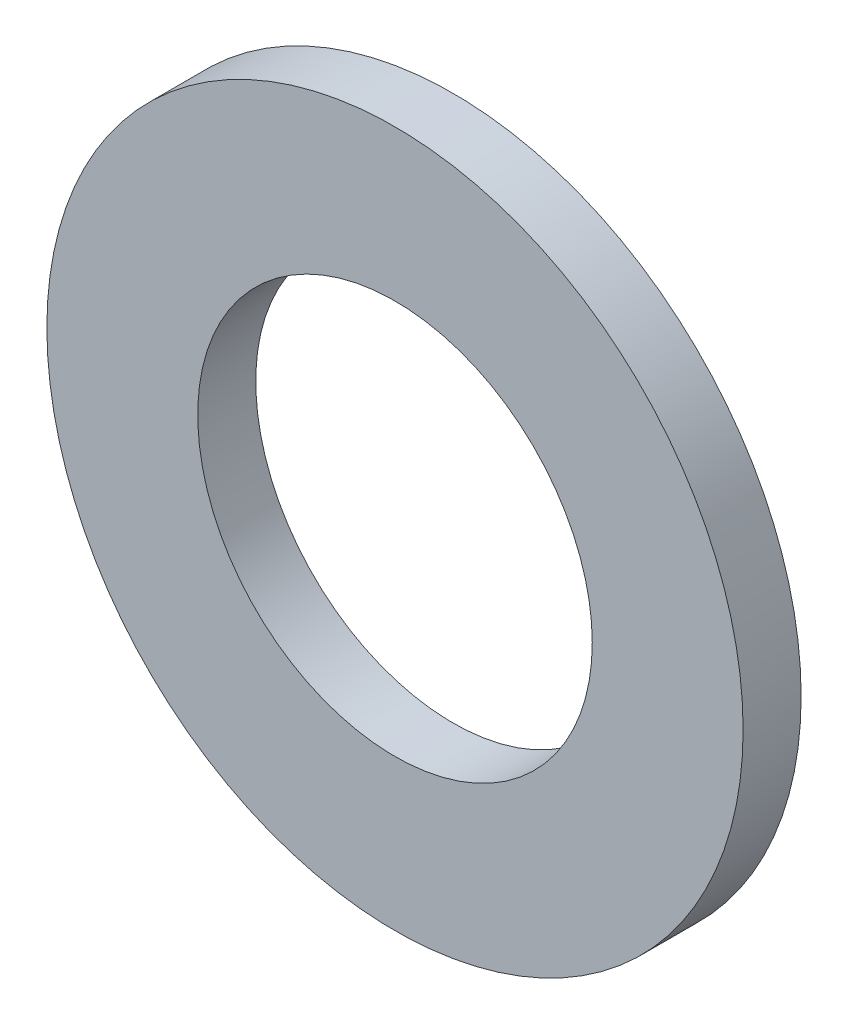
SolidWorks part; units mm, degrees
ref_plane "前视基准面" through (0, 0, 0) normal (0, 0, 1) x (1, 0, 0)
ref_plane "上视基准面" through (0, 0, 0) normal (0, 1, 0) x (1, 0, 0)
ref_plane "右视基准面" through (0, 0, 0) normal (1, 0, 0) x (0, 0, -1)
other "Configuration Table"
sketch "草图1" plane through (0, 0, 0) normal (0, 0, 1) x (1, 0, 0)
  circle A0 centre (0, 0) radius 9
  circle A1 centre (0, 0) radius 5.1
  point P0 (0, 0)
  dimension "D1" = 10.2
  dimension "D2" = 18
extrude "凸台-拉伸1" add sketch "草图1" against normal mid plane 1.5
